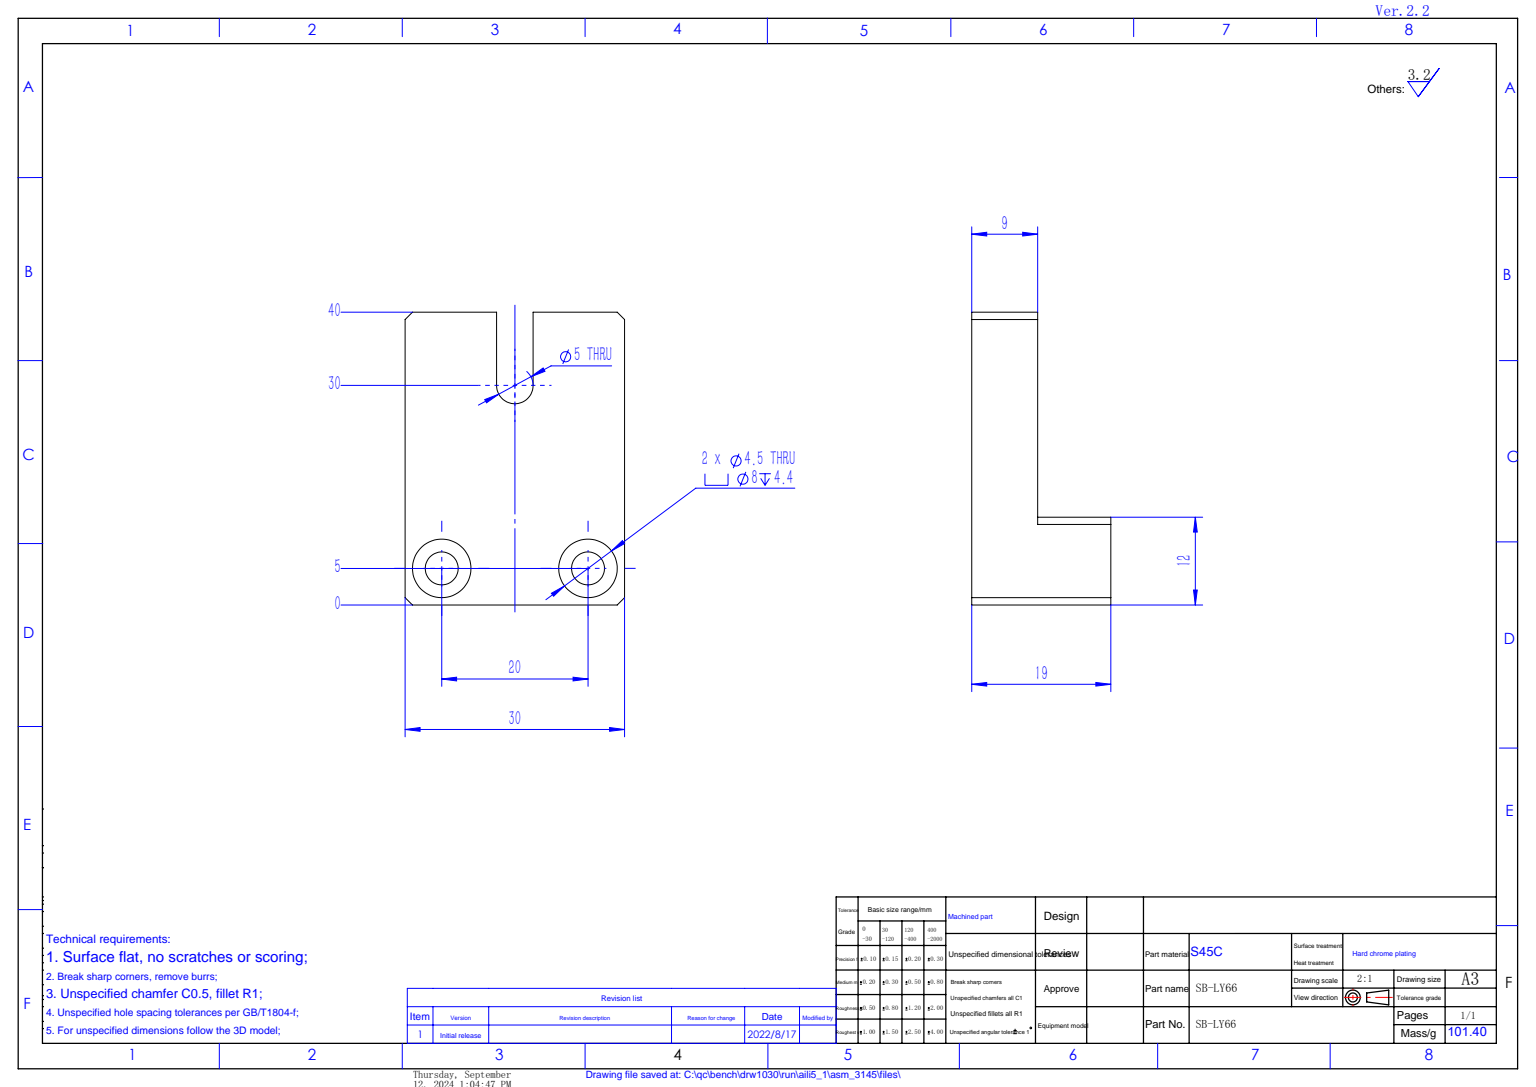
SolidWorks part; units mm, degrees
material "S45C"
ref_plane "前视基准面" through (0, 0, 0) normal (0, 0, 1) x (1, 0, 0)
ref_plane "上视基准面" through (0, 0, 0) normal (0, 1, 0) x (1, 0, 0)
ref_plane "右视基准面" through (0, 0, 0) normal (1, 0, 0) x (0, 0, -1)
sketch "草图1" plane through (0, 0, 0) normal (0, 1, 0) x (1, 0, 0)
  line L1 (15, -20) -> (-15, -20)
  line L2 (15, -20) -> (15, 20)
  line L3 (15, 20) -> (-15, 20)
  line L4 (-15, -20) -> (-15, 20)
  line L5 (15, -20) -> (-15, 20) construction
  line L6 (15, 20) -> (-15, -20) construction
  point P0 (0, 0)
  dimension "D1" = 30
  dimension "D2" = 40
extrude "凸台-拉伸1" add sketch "草图1" along normal blind 9
sketch "草图2" plane through (0, 9, 0) normal (0, 1, 0) x (1, 0, 0)
  line L0 (15, -20) -> (15, 20) construction
  line L1 (-15, 20) -> (15, 20)
  line L2 (-15, 20) -> (-15, 8)
  line L3 (-15, 8) -> (15, 8)
  line L4 (15, 20) -> (15, 8)
  dimension "D1" = 12
extrude "凸台-拉伸2" add sketch "草图2" along normal blind 10
hole_wizard "M4 六角凹头螺钉的柱形沉头孔1" positions "草图3" profile "草图4" counterbore size "M4" standard "ISO" end condition through all
sketch "草图3" plane through (0, 0, 0) normal (0, -1, 0) x (-1, 0, 0)
  line L0 (-10, 15) -> (10, 15) construction
  line L2 (0, 15) -> (0, 20) construction
  line L3 (-15, 20) -> (15, 20) construction
  point P0 (-10, 15)
  point P2 (10, 15)
  dimension "D1" = 20
  dimension "D2" = 5
sketch "草图4" plane through (10, 0, -15) normal (1, 0, 0) x (0, 0, -1)
  line L0 (0, 0) -> (0, 19)
  line L1 (0, 19) -> (2.25, 19)
  line L3 (2.25, 19) -> (2.25, 4.4)
  line L4 (2.25, 4.4) -> (4, 4.4)
  line L5 (4, 4.4) -> (4, 0)
  line L7 (4, 0) -> (0, 0)
  line L11 (0, -6.35) -> (0, 107.95) construction
  dimension "通孔孔直径" = 4.5
  dimension "通孔孔深度" = 19
  dimension "柱形沉头孔直径" = 8
  dimension "柱形沉头孔深度" = 4.4
chamfer "倒角1" distance 1 angle 45 6 edges at (-15, 4.5, 20) (15, 4.5, 20) (-15, 14, -8) (15, 14, -8) (-15, 9.5, -20) (15, 9.5, -20)
sketch "草图5" plane through (0, 0, 0) normal (0, -1, 0) x (1, 0, 0)
  line L0 (0, 20) -> (0, 10) construction
  line L1 (-14, 20) -> (14, 20) construction
  line L2 (2.5, 20) -> (2.5, 10)
  line L3 (-2.5, 20) -> (-2.5, 10)
  arc A0 (2.5, 20) -> (-2.5, 20) centre (0, 20) ccw
  arc A1 (-2.5, 10) -> (2.5, 10) centre (0, 10) ccw
  point P5 (0, 15)
  dimension "D1" = 2.5
  dimension "D2" = 10
extrude "切除-拉伸1" cut sketch "草图5" against normal through all
